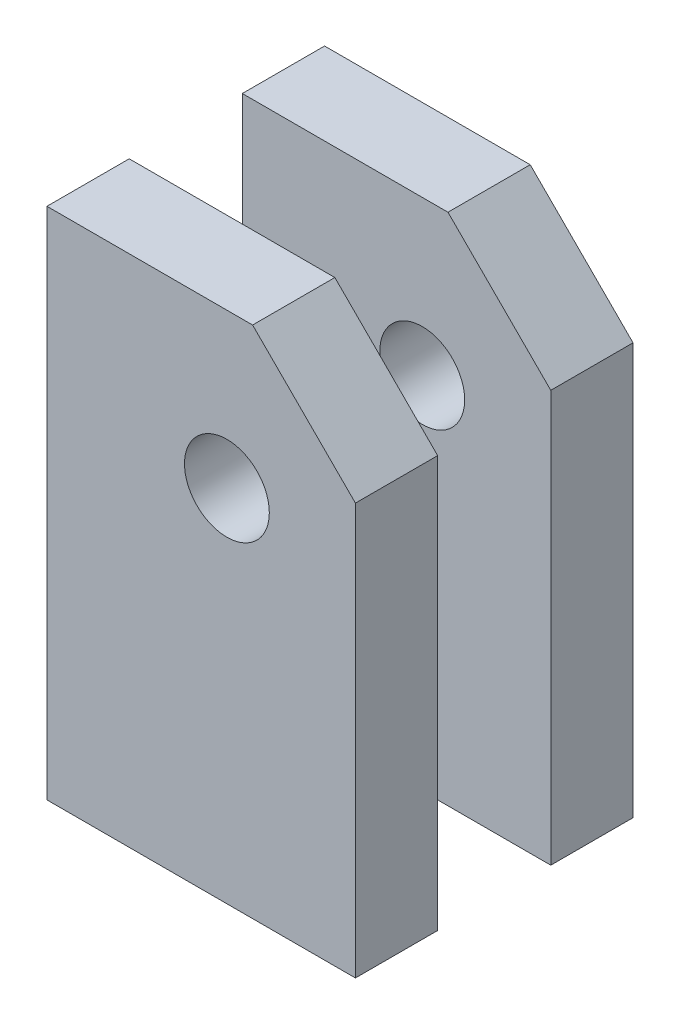
from build123d import *

# Parameters (mm, degrees)
SKETCH1_W           = 60
SKETCH1_H           = 100
BOSS_EXTRUDE1_DEPTH = 16
SKETCH2_R           = 8.25
CUT_EXTRUDE1_DEPTH  = 16
CHAMFER1_SIZE       = 20


with BuildPart() as part:
    # Sketch1 → Boss-Extrude1 (new body)
    with BuildSketch(Plane.XY):
        Rectangle(SKETCH1_W, SKETCH1_H)
    extrude(amount=BOSS_EXTRUDE1_DEPTH)

    # Sketch2 → Cut-Extrude1 (cut)
    with BuildSketch(Plane.XY.offset(16)):
        with Locations((5, 20)):
            Circle(SKETCH2_R)
    extrude(amount=-CUT_EXTRUDE1_DEPTH, mode=Mode.SUBTRACT)

    # Chamfer1
    chamfer1_edges = [part.edges().sort_by_distance(p)[0] for p in [
        (30, 50, 8),
    ]]
    chamfer(chamfer1_edges, length=CHAMFER1_SIZE)


with BuildPart() as body_2:
    # Mirror1: mirrored copy
    add(part.part.mirror(Plane(origin=(0, 0, -11), x_dir=(1, 0, 0), z_dir=(0, 0, -1))))


solid = Compound([part.part, body_2.part])
